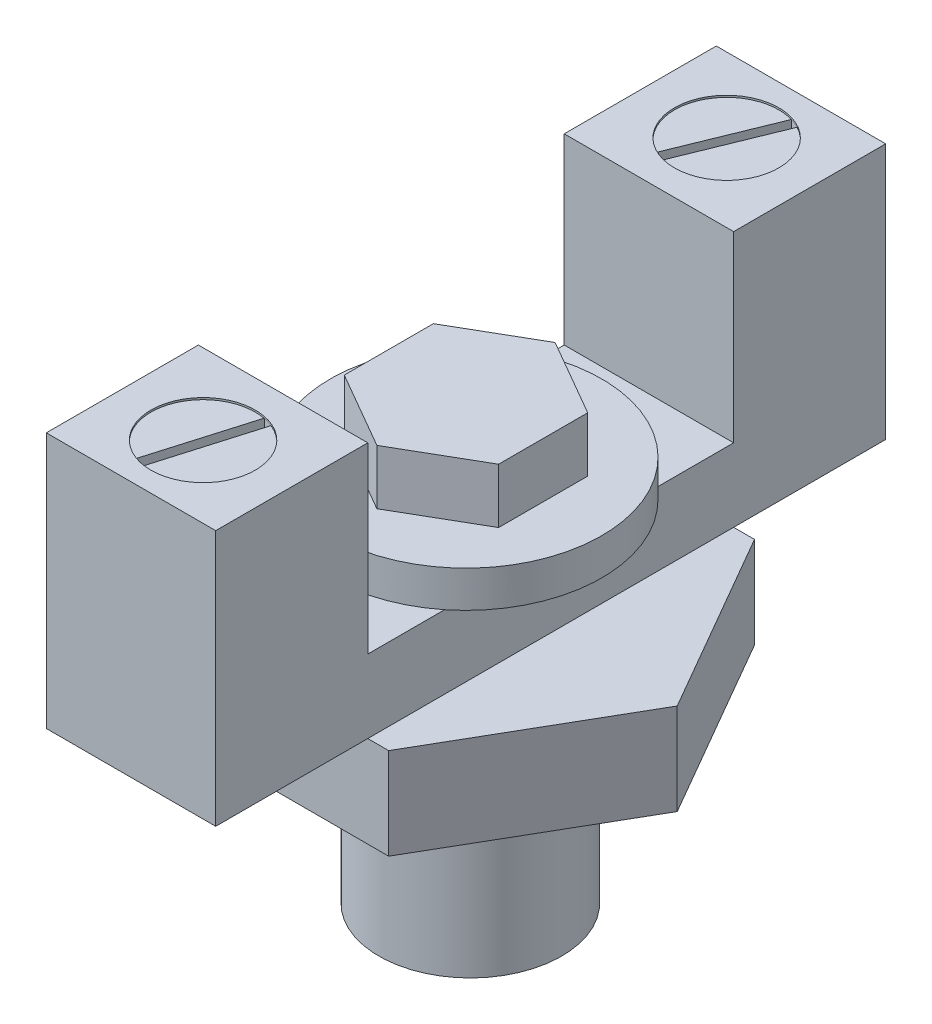
from build123d import *

# Parameters (mm, degrees)
BOSS_EXTRUDE1_DEPTH = 5
SKETCH2_R           = 5
BOSS_EXTRUDE2_DEPTH = 10
SKETCH3_W           = 9.261773254
SKETCH3_H           = 36.627775898
BOSS_EXTRUDE3_DEPTH = 4
SKETCH4_W           = 9.261773254
SKETCH4_H           = 8.313887949
BOSS_EXTRUDE4_DEPTH = 10
SKETCH5_R           = 7.423962758
BOSS_EXTRUDE5_DEPTH = 2
BOSS_EXTRUDE6_DEPTH = 3
SKETCH7_R           = 2.850666807
CUT_EXTRUDE1_DEPTH  = 0.1
CUT_EXTRUDE2_DEPTH  = 1


with BuildPart() as part:
    # Sketch1 → Boss-Extrude1 (new body)
    with BuildSketch(Plane(origin=(0, 0, 0), x_dir=(1, 0, 0), z_dir=(0, 1, 0))):
        Polygon((5.773502692, 10), (-5.773502692, 10), (-11.547005384, 0), (-5.773502692, -10), (5.773502692, -10), (11.547005384, 0), align=None)
    extrude(amount=BOSS_EXTRUDE1_DEPTH)

    # Sketch2 → Boss-Extrude2 (add)
    with BuildSketch(Plane.XZ):
        with Locations(Location((0.234789437, 0, 0), (0, 0, 270))):
            Circle(SKETCH2_R)
    extrude(amount=BOSS_EXTRUDE2_DEPTH)

    # Sketch3 → Boss-Extrude3 (add)
    with BuildSketch(Plane(origin=(0, 5, 0), x_dir=(1, 0, 0), z_dir=(0, 1, 0))):
        Rectangle(SKETCH3_W, SKETCH3_H)
    extrude(amount=BOSS_EXTRUDE3_DEPTH)

    # Sketch4 → Boss-Extrude4 (add)
    with BuildSketch(Plane(origin=(0, 9, 0), x_dir=(1, 0, 0), z_dir=(0, 1, 0))):
        with Locations((0, 14.156943975)):
            Rectangle(SKETCH4_W, SKETCH4_H)
        with Locations((0, -14.156943975)):
            Rectangle(SKETCH4_W, SKETCH4_H)
    extrude(amount=BOSS_EXTRUDE4_DEPTH)

    # Sketch5 → Boss-Extrude5 (add)
    with BuildSketch(Plane(origin=(0, 9, 0), x_dir=(1, 0, 0), z_dir=(0, 1, 0))):
        with Locations(Location((0, 0, 0), (0, 0, 51.407625877))):
            Circle(SKETCH5_R)
    extrude(amount=BOSS_EXTRUDE5_DEPTH)

    # Sketch6 → Boss-Extrude6 (add)
    with BuildSketch(Plane(origin=(0, 11, 0), x_dir=(1, 0, 0), z_dir=(0, 1, 0))):
        Polygon((0, 4.871086868), (-4.218484972, 2.435543434), (-4.218484972, -2.435543434), (0, -4.871086868), (4.218484972, -2.435543434), (4.218484972, 2.435543434), align=None)
    extrude(amount=BOSS_EXTRUDE6_DEPTH)

    # Sketch7 → Cut-Extrude1 (cut)
    with BuildSketch(Plane(origin=(0, 19, 0), x_dir=(1, 0, 0), z_dir=(0, 1, 0))):
        with Locations(Location((0, 14.250511049, 0), (0, 0, 270))):
            Circle(SKETCH7_R)
        with Locations(Location((0, -14.372767949, 0), (0, 0, 270))):
            Circle(SKETCH7_R)
    extrude(amount=-CUT_EXTRUDE1_DEPTH, mode=Mode.SUBTRACT)

    # Sketch8 → Cut-Extrude2 (cut)
    with BuildSketch(Plane(origin=(0, 18.9, 0), x_dir=(1, 0, 0), z_dir=(0, 1, 0))):
        Polygon((-1.343066927, 11.719300444), (0.804329856, 17.000767289), (1.330666503, 16.786763555), (-0.81673028, 11.505296711), align=None)
        Polygon((-1.076876675, -17.027451515), (0.531783037, -11.557769723), (1.076876675, -11.718084383), (-0.531783037, -17.187766175), align=None)
    extrude(amount=-CUT_EXTRUDE2_DEPTH, mode=Mode.SUBTRACT)


solid = part.part
